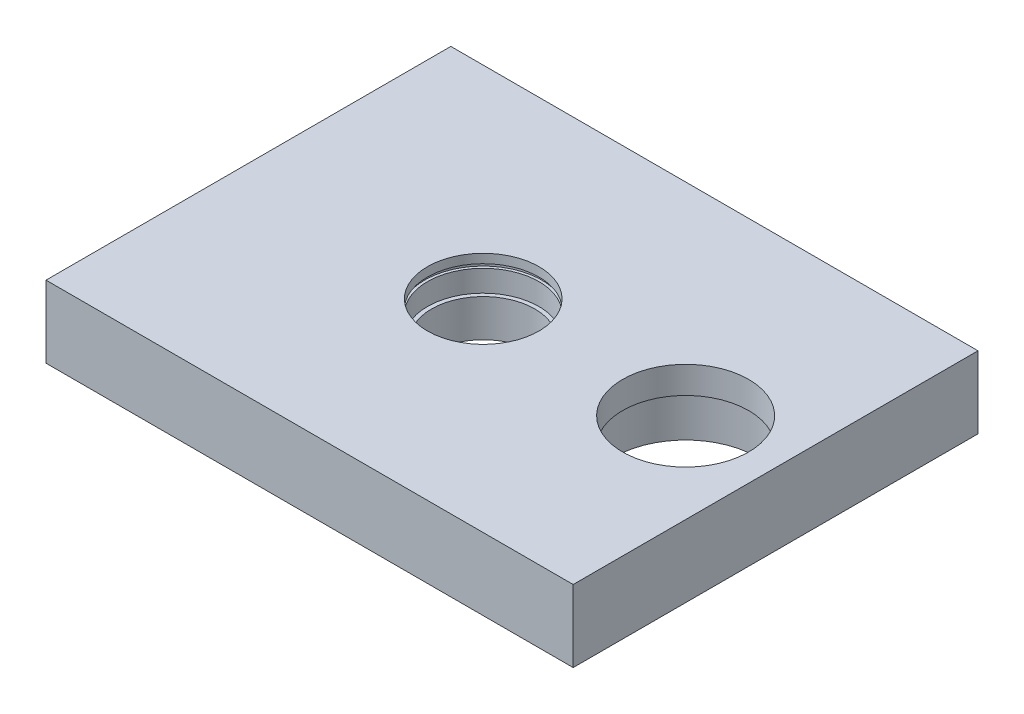
SolidWorks part; units mm, degrees
ref_plane "前视基准面" through (0, 0, 0) normal (0, 0, 1) x (1, 0, 0)
ref_plane "上视基准面" through (0, 0, 0) normal (0, 1, 0) x (1, 0, 0)
ref_plane "右视基准面" through (0, 0, 0) normal (1, 0, 0) x (0, 0, -1)
sketch "草图1" plane through (0, 0, 0) normal (0, 1, 0) x (1, 0, 0)
  line L1 (-146.5, -112.5) -> (146.5, -112.5)
  line L2 (-146.5, -112.5) -> (-146.5, 112.5)
  line L3 (-146.5, 112.5) -> (146.5, 112.5)
  line L4 (146.5, -112.5) -> (146.5, 112.5)
  line L5 (-146.5, -112.5) -> (146.5, 112.5) construction
  line L6 (-146.5, 112.5) -> (146.5, -112.5) construction
  point P0 (0, 0)
  dimension "D1" = 225
  dimension "D2" = 293
extrude "凸台-拉伸1" add sketch "草图1" along normal blind 40
sketch "草图2" plane through (0, 0, 0) normal (0, -1, 0) x (1, 0, 0)
  line L0 (146.5, 112.5) -> (146.5, -112.5) construction
  line L1 (-146.5, 112.5) -> (146.5, 112.5) construction
  circle A0 centre (96.5, 0) radius 40
  dimension "D1" = 80
  dimension "D2" = 50
  dimension "D3" = 112.5
extrude "切除-拉伸1" cut sketch "草图2" against normal blind 25
sketch "草图3" plane through (0, 0, 0) normal (0, -1, 0) x (1, 0, 0)
  line L0 (146.5, 112.5) -> (146.5, -112.5) construction
  line L1 (-146.5, 112.5) -> (146.5, 112.5) construction
  circle A0 centre (-16, 0) radius 28.7
  dimension "D1" = 57.4
  dimension "D2" = 162.5
  dimension "D3" = 112.5
extrude "切除-拉伸2" cut sketch "草图3" against normal through all
sketch "草图4" plane through (0, 0, 0) normal (0, -1, 0) x (1, 0, 0)
  line L0 (146.5, 112.5) -> (146.5, -112.5) construction
  circle A0 centre (96.5, 0) radius 35
  dimension "D1" = 70
  dimension "D2" = 50
  dimension "D3" = 112.5
extrude "切除-拉伸3" cut sketch "草图4" against normal through all
sketch "草图5" plane through (0, 40, 0) normal (0, 1, 0) x (1, 0, 0)
  circle A0 centre (-16, 0) radius 31
  dimension "D1" = 62
extrude "切除-拉伸4" cut sketch "草图5" against normal blind 19.2
ref_plane "基准面1" through (0, 35, 0) normal (0, 1, 0) x (1, 0, 0)
sketch "草图6" plane through (0, 35, 0) normal (0, 1, 0) x (1, 0, 0)
  circle A0 centre (-16, 0) radius 32.5
  dimension "D1" = 65
extrude "切除-拉伸5" cut sketch "草图6" against normal blind 2.2
